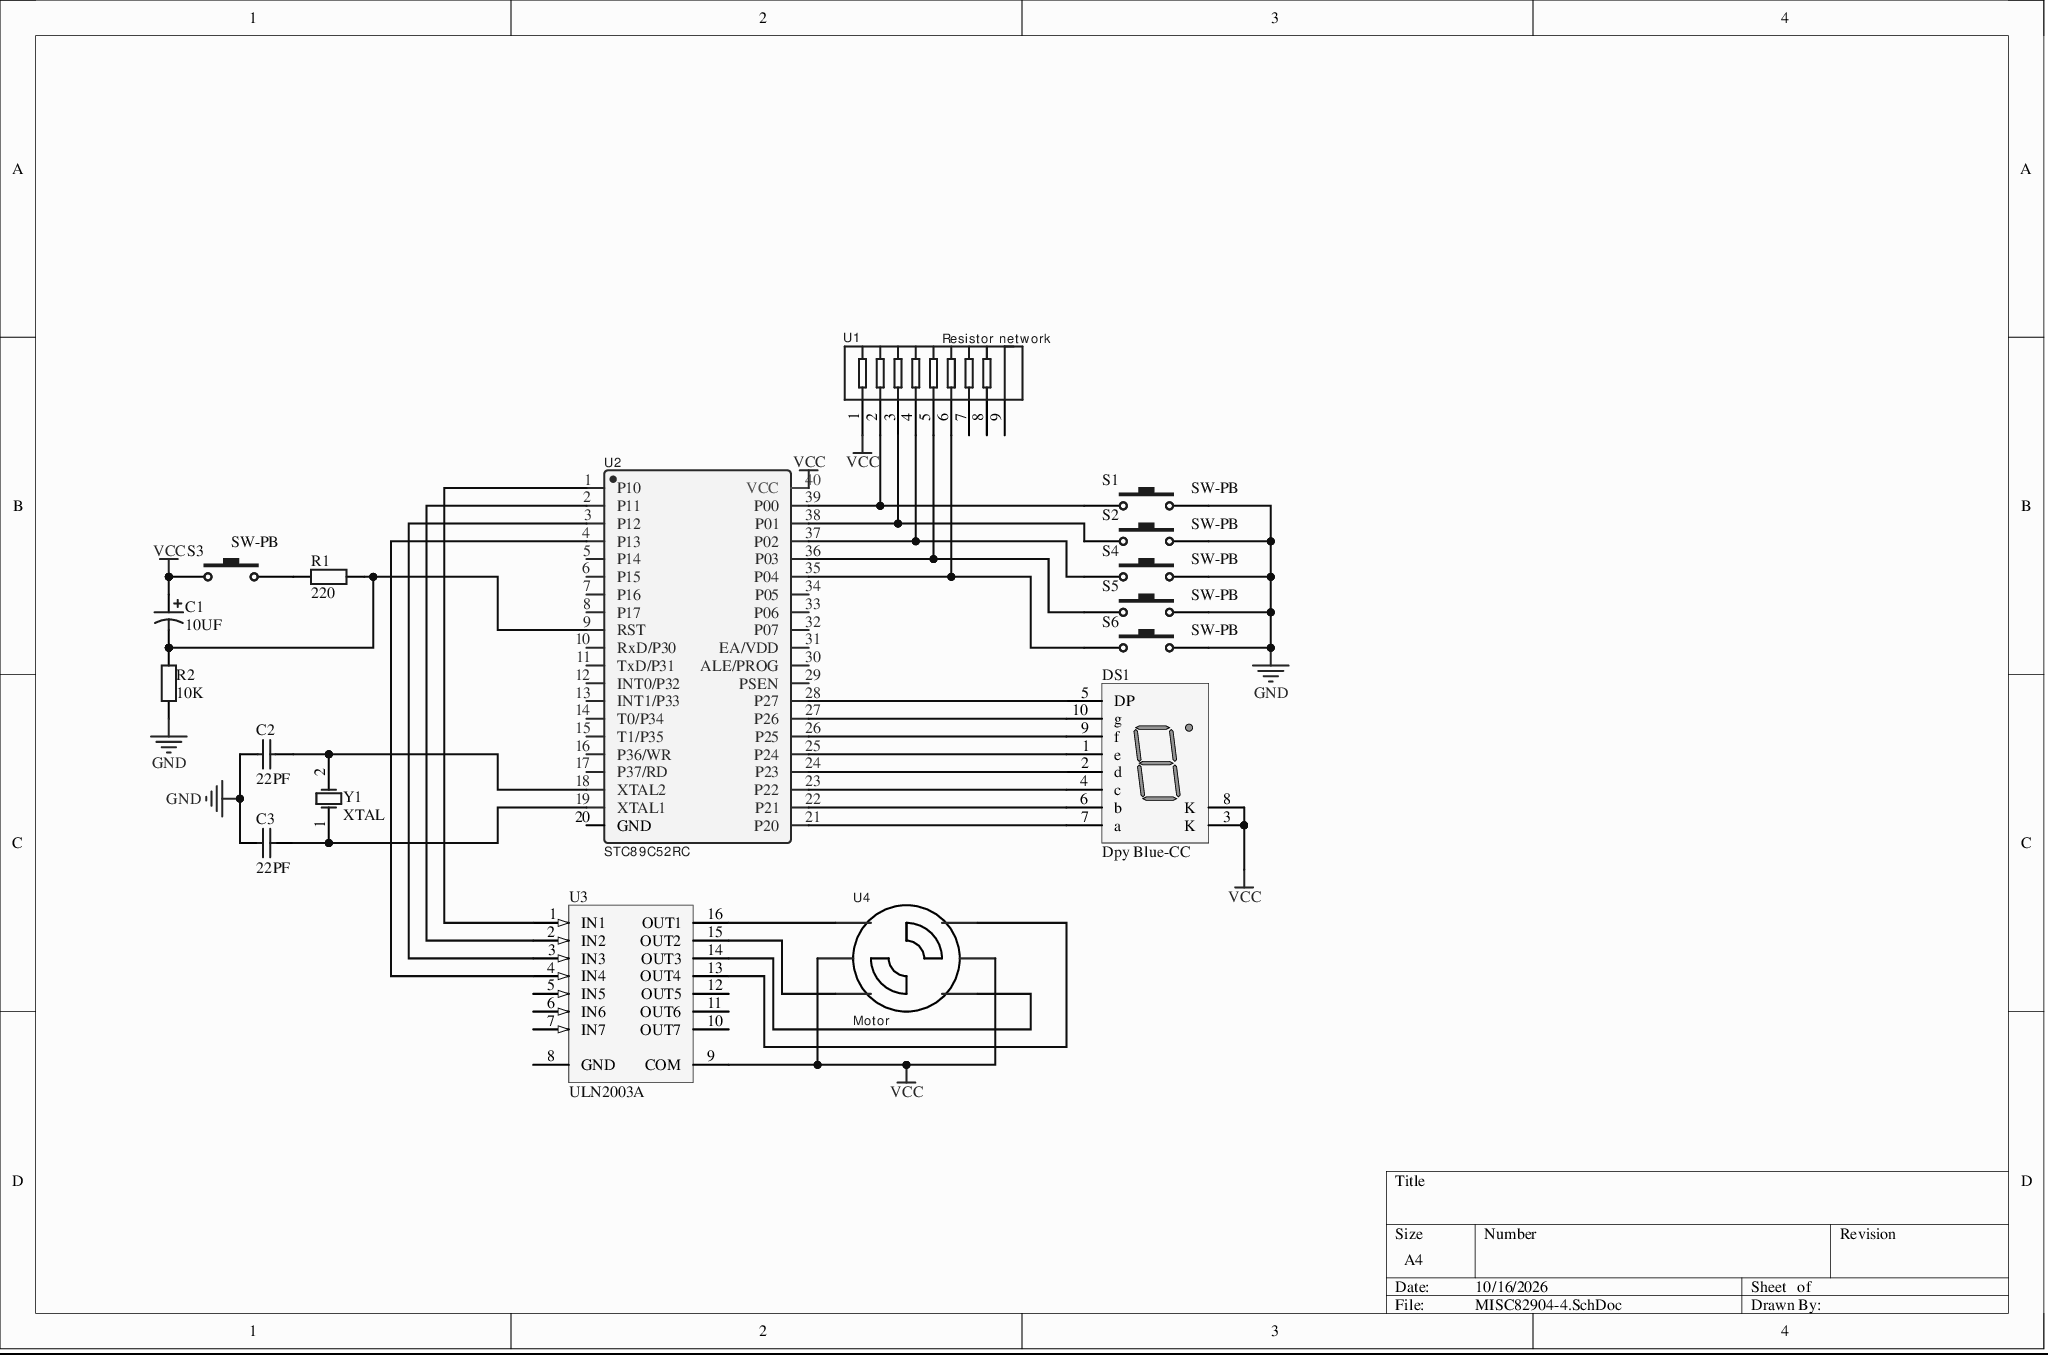
[diagram p0: MISC82904-4.SchDoc]
# Altium project MISC82904-7.PrjPcb
1 sheet, 17 parts. Net scope: global (net labels, ports and power ports of the same name join across sheets).
Board file: MISC82904.PcbDoc

## Sheet MISC82904-4.SchDoc
size A4

### Parts
C1  10UF  [RB7.6-15]
C2  22PF  [RAD-0.3]
C3  22PF  [RAD-0.3]
DS1  Dpy Blue-CC  [H]
R1  220  [AXIAL-0.4]
R2  10K  [AXIAL-0.4]
S1  SW-PB  [SPST-2]
S2  SW-PB  [SPST-2]
S3  SW-PB  [SPST-2]
S4  SW-PB  [SPST-2]
S5  SW-PB  [SPST-2]
S6  SW-PB  [SPST-2]
U1  Resistor network  [paizu]
U2  STC89C52RC  [STC89C52RC]
U3  ULN2003A  [A16]
U4  Motor  [HDR1X6]
Y1  XTAL  [R38]

### Nets
GND: C2.1 C3.1 R2.1 S1.2 S2.2 S4.2 S5.2 S6.2
VCC: C1.1 DS1.3(K) DS1.8(K) S3.1 U1.1 U2.40(VCC) U3.9(COM) U4.3 U4.5
NetC1_2: C1.2 R1.1 R2.2 U2.9(RST)
NetC2_2: C2.2 U2.18(XTAL2) Y1.2(OSC2)
NetC3_2: C3.2 U2.19(XTAL1) Y1.1(OSC1)
NetDS1_1: DS1.1(e) U2.25(P24)
NetDS1_2: DS1.2(d) U2.24(P23)
NetDS1_4: DS1.4(c) U2.23(P22)
NetDS1_5: DS1.5(DP) U2.28(P27)
NetDS1_6: DS1.6(b) U2.22(P21)
NetDS1_7: DS1.7(a) U2.21(P20)
NetDS1_9: DS1.9(f) U2.26(P25)
NetDS1_10: DS1.10(g) U2.27(P26)
NetR1_2: R1.2 S3.2
NetS1_1: S1.1 U1.2 U2.39(P00)
NetS2_1: S2.1 U1.3 U2.38(P01)
NetS4_1: S4.1 U1.4 U2.37(P02)
NetS5_1: S5.1 U1.5 U2.36(P03)
NetS6_1: S6.1 U1.6 U2.35(P04)
NetU2_1: U2.1(P10) U3.1(IN1)
NetU2_2: U2.2(P11) U3.2(IN2)
NetU2_3: U2.3(P12) U3.3(IN3)
NetU2_4: U2.4(P13) U3.4(IN4)
NetU3_13: U3.13(OUT4) U4.4
NetU3_14: U3.14(OUT3) U4.6
NetU3_15: U3.15(OUT2) U4.2
NetU3_16: U3.16(OUT1) U4.1

Not connected (* = marked no-connect by the designer): U1 7 8 9; U2 5(P14) 6(P15) 7(P16) 8(P17) 10(RxD/P30) 11(TxD/P31) 12(INT0/P32) 13(INT1/P33) 14(T0/P34) 15(T1/P35) 16(P36/WR) 17(P37/RD) 20(GND) 29(PSEN) 30(ALE/PROG) 31(EA/VDD) 32(P07) 33(P06) 34(P05); U3 5(IN5) 6(IN6) 7(IN7) 8(GND) 10(OUT7) 11(OUT6) 12(OUT5)

### Library data of the parts
C1 = Cap Pol1: Polarized Capacitor (Radial); Value: 100pF; Published: 8-Jun-2000; LatestRevisionDate: 17-Jul-2002; LatestRevisionNote: Re-released for DXP Platform.; PackageReference: RB7.6-15; PackageDescription: Polarized Capacitor (Radial); 2 Leads; Publisher: Altium Limited
C2 C3 = Cap: Capacitor; Value: 100pF; Published: 8-Jun-2000; LatestRevisionDate: 17-Jul-2002; LatestRevisionNote: Re-released for DXP Platform.; PackageReference: RAD-0.3; PackageDescription: Radial Cap, Thru-Hole; 2 Leads; 0.3 in Pin Spacing; Publisher: Altium Limited
DS1 = Dpy Blue-CC: 14.2 mm General Purpose Blue 7-Segment Display: CC, RH DP, Gray Surface; MinimumIntensity: 2020 ucd; Note: IF = 10 mA; Published: 8-Jun-2000; LatestRevisionDate: 17-Dec-2003; LatestRevisionNote: Schematic revised, PCB Footprint replaced.; DatasheetVersion: 24-Sep-2002; PackageVersion: 24-Sep-2002; PackageReference: H; PackageDescription: LED, 7-Segment Display, 14.2 mm, RHD; 10 Leads; Row Space 15.24 mm; Pitch 2.54 mm; Colour: Blue; ComponentLink1Description: Manufacturer Link; Publisher: Altium Limited
R1 R2 = Res2: Resistor; Value: 1K; Published: 8-Jun-2000; LatestRevisionDate: 17-Jul-2002; LatestRevisionNote: Re-released for DXP Platform.; PackageReference: AXIAL-0.4; PackageDescription: Axial Device, Thru-Hole; 2 Leads; 0.4 in Pin Spacing; Publisher: Altium Limited
S1-S6 = SW-PB: Switch; Published: 24-Mar-1999; LatestRevisionDate: 17-Jul-2002; LatestRevisionNote: Re-released for DXP Platform.; PackageReference: SPST-2; PackageDescription: Switch; 2 Leads; Publisher: Altium Limited
U1 = 排阻
U3 = ULN2003A: High-Voltage, High-Current Darlington Array; Package Information: Latest Revision: 1998; Code - JEDEC: MS-001-BB; Published: 13-Oct-2000; Revision: 17-Jul-2002: Re-released for DXP Platform.; Datasheet: Latest Revision: 1998; Package Reference: A16; Publisher: Altium Limited
U4 = 电机
Y1 = XTAL: Crystal Oscillator; Published: 8-Jun-2000; LatestRevisionDate: 17-Jul-2002; LatestRevisionNote: Re-released for DXP Platform.; PackageReference: R38; PackageDescription: Crystal, Thru-Hole; 2 Leads; Body 3.1 x 8.2 mm (Dia.xH); Publisher: Altium Limited